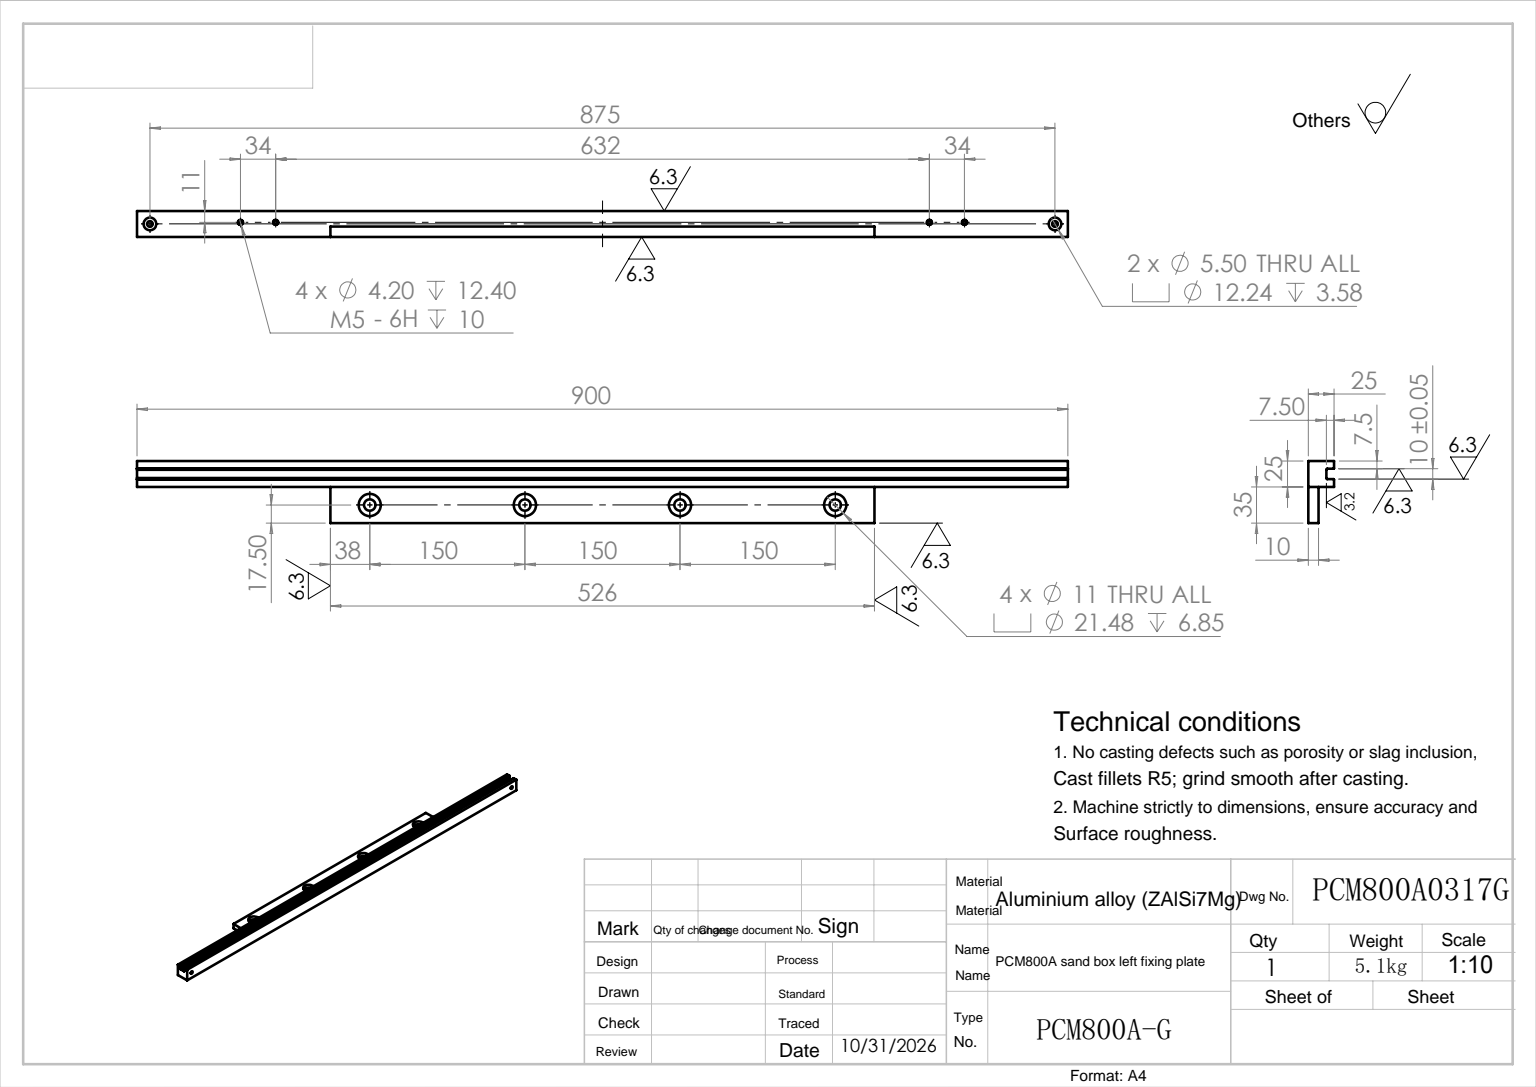
SolidWorks part; units mm, degrees
ref_plane "前视" through (0, 0, 0) normal (0, 0, 1) x (1, 0, 0)
ref_plane "上视" through (0, 0, 0) normal (0, 1, 0) x (1, 0, 0)
ref_plane "右视" through (0, 0, 0) normal (1, 0, 0) x (0, 0, -1)
sketch "草图1" plane through (0, 0, 0) normal (1, 0, 0) x (0, 0, -1)
  line L1 (0, 0) -> (900, 0)
  line L2 (0, 0) -> (0, 25)
  line L3 (0, 25) -> (900, 25)
  line L4 (900, 0) -> (900, 25)
  dimension "D1" = 25
  dimension "D2" = 900
extrude "拉伸1" add sketch "草图1" along normal blind 25
sketch "草图2" plane through (0, 0, 0) normal (-1, 0, 0) x (0, 0, 1)
  line L0 (0, 0) -> (-900, 0) construction
  line L1 (-713, 0) -> (-187, 0)
  line L2 (-713, 0) -> (-713, 10)
  line L3 (-713, 10) -> (-187, 10)
  line L4 (-187, 0) -> (-187, 10)
  dimension "D1" = 10
  dimension "D2" = 526
  dimension "D3" = 187
extrude "拉伸2" add sketch "草图2" along normal blind 35
sketch "草图3" plane through (0, 0, 0) normal (0, 0, 1) x (1, 0, 0)
  line L0 (25, 25) -> (0, 25) construction
  line L1 (7.5, 25) -> (17.5, 25)
  line L2 (7.5, 25) -> (7.5, 18.5)
  line L3 (8.5, 17.5) -> (16.5, 17.5)
  line L4 (17.5, 25) -> (17.5, 18.5)
  arc A0 (8.5, 17.5) -> (7.5, 18.5) centre (8.5, 18.5) cw
  arc A1 (17.5, 18.5) -> (16.5, 17.5) centre (16.5, 18.5) cw
  point P9 (7.5, 17.5)
  dimension "D4" = 1
  dimension "D1" = 10
  dimension "D2" = 7.5
  dimension "D3" = 7.5
extrude "切除-拉伸1" cut sketch "草图3" against normal through all
chamfer "倒角1" distance 0.5 angle 45 2 edges at (17.5, 25, -450) (7.5, 25, -450)
sketch "草图4" plane through (0, 10, 0) normal (0, 1, 0) x (-1, 0, 0)
  line L0 (17.5, -713) -> (17.5, -187) construction
  line L1 (35, -713) -> (0, -713) construction
  line L2 (35, -187) -> (0, -187) construction
  line L3 (17.5, -675) -> (35, -675) construction
  line L4 (35, -187) -> (35, -713) construction
  line L5 (17.5, -525) -> (35, -525) construction
  line L6 (17.5, -375) -> (35, -375) construction
  line L7 (17.5, -225) -> (35, -225) construction
  dimension "D1" = 38
  dimension "D2" = 150
  dimension "D3" = 150
  dimension "D4" = 150
hole_wizard "M10 六角头螺栓的柱形沉头孔1" positions "3D草图1" profile "草图5" counterbore size "M10" standard "Ansi Metric" end condition through all
sketch3d "3D草图1"
  line L1 (-35, 10, -713) -> (0, 10, -713) construction
  line L3 (-35, 10, -187) -> (0, 10, -187) construction
  line L4 (-35, 10, -187) -> (-35, 10, -713) construction
  point P19 (-17.5, 10, -675)
  point P21 (-17.5, 10, -525)
  point P23 (-17.5, 10, -375)
  point P25 (-17.5, 10, -225)
  dimension "D1" = 38
  dimension "D2" = 150
  dimension "D3" = 150
  dimension "D4" = 150
  dimension "D5" = 38
  dimension "D6" = 17.5
sketch "草图5" plane through (-17.5, 10, -675) normal (1, 0, 0) x (0, 0, 1)
  line L0 (0, 0) -> (0, 10)
  line L1 (0, 10) -> (5.5, 10)
  line L3 (5.5, 10) -> (5.5, 6.85)
  line L4 (5.5, 6.85) -> (10.74, 6.85)
  line L5 (10.74, 6.85) -> (10.74, 0)
  line L7 (10.74, 0) -> (0, 0)
  line L11 (0, -6.35) -> (0, 107.95) construction
  dimension "籵謂謂眻噤" = 11
  dimension "籵謂謂旮僅" = 10
  dimension "翐倛麥芛謂眻噤" = 21.48
  dimension "翐倛麥芛謂旮僅" = 6.85
sketch "草图6" plane through (0, 0, 0) normal (-1, 0, 0) x (0, 0, 1)
  line L0 (-900, 12.5) -> (0, 12.5) construction
  line L1 (-900, 0) -> (-900, 25) construction
  line L2 (0, 25) -> (0, 0) construction
  line L3 (-12.5, 12.5) -> (-12.5, 25) construction
  line L4 (-900, 25) -> (0, 25) construction
  line L5 (-887.5, 25) -> (-887.5, 12.5) construction
  dimension "D1" = 12.5
  dimension "D2" = 12.5
hole_wizard "M5 六角头螺栓的柱形沉头孔1" positions "3D草图2" profile "草图7" counterbore size "M5" standard "Ansi Metric" end condition through all
sketch3d "3D草图2"
  line L2 (0, 25, -900) -> (0, 25, 0) construction
  line L3 (0, 0, -900) -> (0, 25, -900) construction
  line L4 (0, 25, 0) -> (0, 0, 0) construction
  point P10 (0, 12.5, -887.5)
  point P12 (0, 12.5, -12.5)
  dimension "D1" = 12.5
  dimension "D2" = 12.5
  dimension "D3" = 12.5
  dimension "D4" = 12.5
sketch "草图7" plane through (0, 12.5, -887.5) normal (0, 1, 0) x (0, 0, 1)
  line L0 (0, 0) -> (0, 25)
  line L1 (0, 25) -> (2.75, 25)
  line L3 (2.75, 25) -> (2.75, 3.58)
  line L4 (2.75, 3.58) -> (6.12, 3.58)
  line L5 (6.12, 3.58) -> (6.12, 0)
  line L7 (6.12, 0) -> (0, 0)
  line L11 (0, -6.35) -> (0, 107.95) construction
  dimension "籵謂謂眻噤" = 5.5
  dimension "籵謂謂旮僅" = 25
  dimension "翐倛麥芛謂眻噤" = 12.24
  dimension "翐倛麥芛謂旮僅" = 3.58
hole_wizard "M5 螺纹孔1" positions "3D草图3" profile "草图8" tap size "M5" standard "GB"
sketch3d "3D草图3"
  line L0 (0, 25, -900) -> (0, 25, 0) construction
  line L1 (0, 0, -900) -> (0, 25, -900) construction
  point P0 (0, 14, -800)
  point P2 (0, 14, -766)
  dimension "D1" = 34
  dimension "D2" = 11
  dimension "D3" = 11
  dimension "D4" = 100
sketch "草图8" plane through (0, 14, -800) normal (0, 1, 0) x (0, 0, 1)
  line L0 (0, 0) -> (0, 13.6618)
  line L1 (0, 13.6618) -> (2.1, 12.4)
  line L2 (2.1, 12.4) -> (2.1, 10)
  line L3 (2.1, 10) -> (2.5, 10)
  line L4 (2.5, 10) -> (2.5, 0)
  line L5 (2.5, 0) -> (0, 0)
  line L10 (0, 13.6618) -> (-2.1, 12.4) construction
  line L11 (0, -6.35) -> (0, 107.95) construction
  dimension "螺纹孔钻头直径" = 4.2
  dimension "螺纹孔钻头深度" = 12.4
  dimension "螺纹主直径" = 5
  dimension "螺纹深度" = 10
  dimension "导头角度" = 118
pattern_linear "阵列(线性)1" count 2 spacing 666 along (0, 0, 1) of "M5 螺纹孔1"
